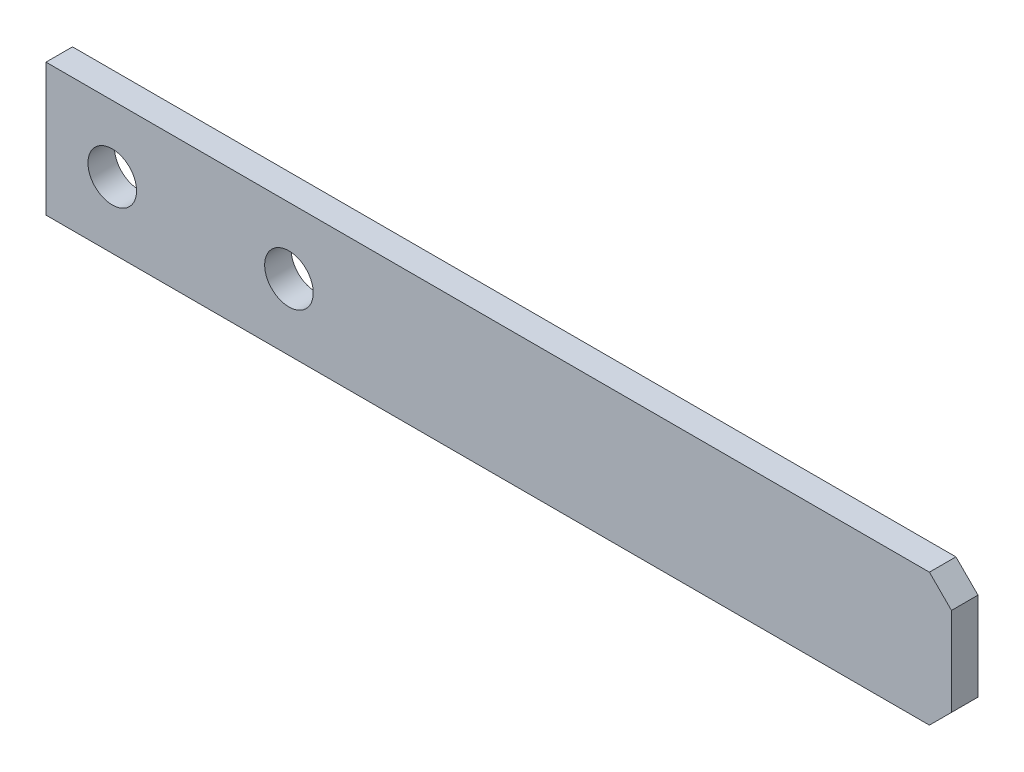
SolidWorks part; units mm, degrees
material "1023 碳钢板 (SS)"
ref_plane "Front Plane" through (0, 0, 0) normal (0, 0, 1) x (1, 0, 0)
ref_plane "Top Plane" through (0, 0, 0) normal (0, 1, 0) x (1, 0, 0)
ref_plane "Right Plane" through (0, 0, 0) normal (1, 0, 0) x (0, 0, -1)
ref_plane "Plane4" through (0, 0, 3) normal (0, 0, 1) x (1, 0, 0)
sketch "Sketch1" plane through (0, 0, 3) normal (0, 0, 1) x (1, 0, 0)
  line L0 (102.5, -10) -> (102.5, 10)
  line L1 (102.5, 10) -> (97.5, 15)
  line L2 (97.5, 15) -> (-102.5, 15)
  line L3 (-102.5, 15) -> (-102.5, -15)
  line L4 (-102.5, -15) -> (97.5, -15)
  line L5 (97.5, -15) -> (102.5, -10)
  circle A0 centre (-87.5, 0) radius 5.5
  circle A1 centre (-47.5, 0) radius 5.5
extrude "Boss-Extrude1" add sketch "Sketch1" against normal blind 6
